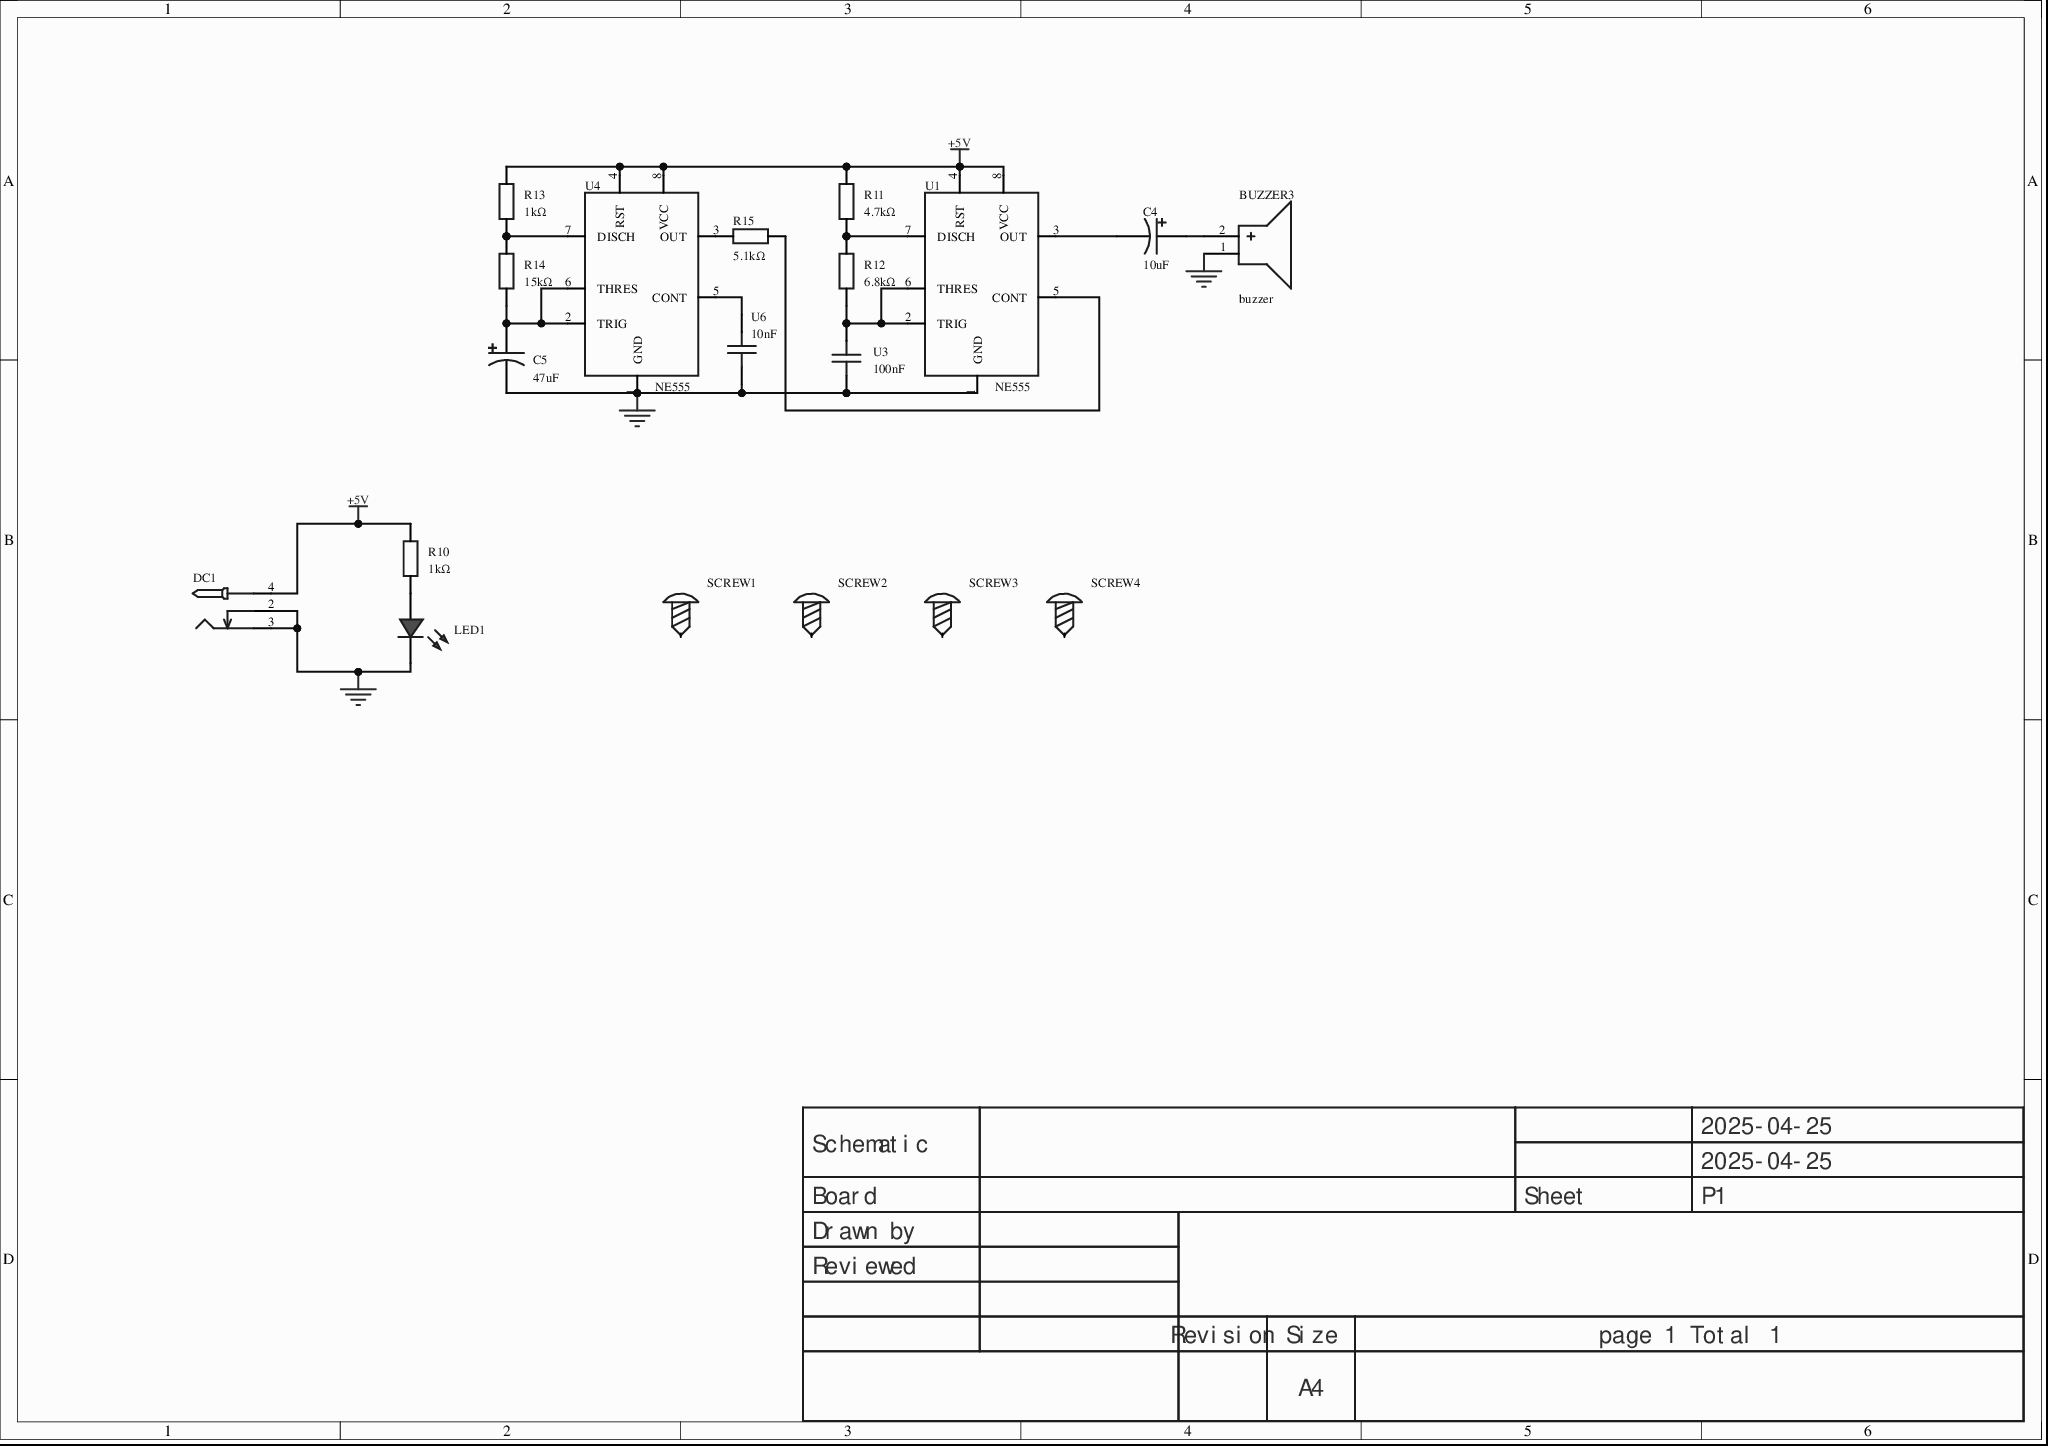
[diagram p0: MISC51829-3.schdoc]
# Altium project MISC51829-2.PrjPcb
1 sheet, 19 parts. Net scope: global (net labels, ports and power ports of the same name join across sheets).
Board file: MISC51829.pcbdoc

## Sheet MISC51829-3.schdoc
size 297 x 209 mm; Version: V1.0; @Project Name: MISC51829; @Page Count: 1; @Update Date: 2025-04-25; @Create Date: 2025-04-25; @Schematic Name: MISC51829; @Page No: 1; @Create Time: 10:10:14; @Update Time: 10:10:18; @Board Name: MISC51829

### Parts
BUZZER3  buzzer  [BUZ-TH_BD12.0-P6.00-D0.9-RD]
C4  10uF  [CAP-TH_BD5.0-P2.00-D0.8-FD]
C5  47uF  [CAP-TH_BD5.0-P2.00-D0.8-FD]
DC1  (no value)  [DC-2.0]
LED1  (no value)  [LED_TH-3mm]
R10  1kΩ  [Res_1/8W]
R11  4.7kΩ  [Res_1/8W]
R12  6.8kΩ  [Res_1/8W]
R13  1kΩ  [Res_1/8W]
R14  15kΩ  [Res_1/8W]
R15  5.1kΩ  [Res_1/8W]
SCREW1  (no value)  [M3螺丝]
SCREW2  (no value)  [M3螺丝]
SCREW3  (no value)  [M3螺丝]
SCREW4  (no value)  [M3螺丝]
U1  NE555  [PDIP-8_L9.6-W6.4-P2.54-LS7.9-BL-1]
U3  100nF  [CAP-TH_L4.0-W2.5-P2.50-D0.5]
U4  NE555  [PDIP-8_L9.6-W6.4-P2.54-LS7.9-BL-1]
U6  10nF  [CAP-TH_L4.0-W2.5-P2.50-D0.5]

### Nets
+5V: DC1.4 R10.2 R11.2 R13.2 U1.4(RST) U1.8(VCC) U4.4(RST) U4.8(VCC)
GND: BUZZER3.1(-) C5.2 DC1.2 DC1.3 LED1.2(A) U1.1(GND) U3.1 U4.1(GND) U6.1
NetBUZZER3_2: BUZZER3.2(+) C4.1
NetC4_2: C4.2 U1.3(OUT)
NetC5_1: C5.1 R14.1 U4.2(TRIG) U4.6(THRES)
NetLED1_1: LED1.1(C) R10.1
NetR11_1: R11.1 R12.2 U1.7(DISCH)
NetR12_1: R12.1 U1.2(TRIG) U1.6(THRES) U3.2
NetR13_1: R13.1 R14.2 U4.7(DISCH)
NetR15_1: R15.1 U1.5(CONT)
NetR15_2: R15.2 U4.3(OUT)
NetU4_5: U4.5(CONT) U6.2

Not connected (* = marked no-connect by the designer): SCREW1 1; SCREW2 1; SCREW3 1; SCREW4 1

### Notes on the sheet
- 2025-04-25
- Schematic
- Board
- Sheet
- P1
- Drawn by
- Reviewed
- Revision
- Size
- A4
- page 1 Total 1

### Library data of the parts
BUZZER3 = buzzer: AddInBom: yes; ModelId: af17e4151ed84fc2a628230bf2376363; ModelTransform: 472.44,472.176,0,270,0,0,0,0,-196.85; Symbol: BUZZER; Device: buzzer; LCSC Part Name: buzzer; SupplierPart: C9900014030; ManufacturerPart: buzzer; Supplier Footprint: buzzer; JLCPCB Part Class: Extended library; Supplier: LCSC; ConvertToPcb: yes; FootprintName: BUZ-TH_BD12.0-P6.00-D0.9-RD; ModelName: BUZ-TH_BD12.0-P6.00-D0.9-RD
C4 C5 = KM475M100D11RR0VH2FP0: Capacitance: 4.7uF; Tolerance: ±20%; Rated voltage: 100V;; Manufacturer: CX(承兴); Symbol: 4.7uF 100V 5*11; AddInBom: yes; ModelId: edeeed87cbc746108d01291548c38636; ModelName: CAP-TH_D5.0×H7.0×P2.0; ModelTransform: 197.091,196.7911,0,0,0,0,0,0,-137.795; φD: 5mm; L: 11mm; Device: KM475M100D11RR0VH2FP0; LCSC Part Name: 4.7uF ±20% 100V; ManufacturerPart: KM475M100D11RR0VH2FP0; Supplier Footprint: 插件,D5xL11mm; JLCPCB Part Class: Extended library; Datasheet: https://atta.szlcsc.com/upload/public/pdf/source/20211027/06D6BA3719C264B639DC286D935D03EA.pdf; Supplier: LCSC; ConvertToPcb: yes; FootprintName: CAP-TH_BD5.0-P2.00-D0.8-FD; Rated Voltage: 100V; Lead Spacing: 2mm; Lifetime @ Temp: -
  C4: Value: 10uF
  C5: Value: 47uF
DC1 = DC-005_2.0: ConvertToPcb: yes; SymbolName: DC power jack; ModelId: f5f20b8a2308479b936ba3c2698865bb0819f05c4eef4c71ace90d822a990e87; ModelName: DC-IN-TH_DC-5520-1; ModelTransform: 372.05,551.18,582.68,90,0,0,137.8,0,-149.61; Device: DC-005_2.0; AddInBom: yes; Supplier Footprint: 插件; FootprintName: DC-2.0
LED1 = LED_TH-R_3mm: ConvertToPcb: yes; ModelId: a497c992633541038a38947cdc58012f; ModelName: LED-TH-3mm_R; ModelTransform: 141.274,153.327,0,0,0,0,-5.984,0,-137.795; Symbol: LED_TH-R; Device: LED_TH-R_3mm; AddInBom: yes; FootprintName: LED_TH-3mm; Supplier Footprint: 插件
R10-R15 = Res_AXIAL-1/8W: ConvertToPcb: yes; SymbolName: Resistor; ModelId: b2b5ae7ae4c642178fe0039925c86a3f; ModelName: RES-TH_BD1.8-L3.2-P7.20-D0.4; ModelTransform: 282.86,66.88,253.09,0,0,0,0,0,-191; Device: Res_AXIAL-1/8W; AddInBom: yes; Supplier Footprint: 轴向引线; FootprintName: Res_1/8W
  R10 R13: Value: 1kΩ
  R11: Value: 4.7kΩ
  R12: Value: 6.8kΩ
  R14: Value: 15kΩ
  R15: Value: 5.1kΩ
SCREW1-SCREW4 = M3螺丝: Device: M3 screw; ConvertToPcb: yes; SymbolName: Screw hole; AddInBom: yes; Supplier Footprint: 插件; FootprintName: M3 screw
U1 U4 = NE555PE4: NE555 single timer; Manufacturer: TI(德州仪器); AddInBom: yes; ModelId: 1b8eaf096e7944deafe216467068c10e; ModelTransform: 377.952,318.897,0,0,0,0,0,0,-118.11; Manufacturer Part: NE555; Symbol: NE555PE4; Device: NE555PE4; LCSC Part Name: NE555PE4; SupplierPart: C2859604; Supplier Footprint: PDIP-8; JLCPCB Part Class: Extended library; Datasheet: https://www.ti.com/cn/lit/gpn/sa555; Supplier: LCSC; ConvertToPcb: yes; FootprintName: PDIP-8_L9.6-W6.4-P2.54-LS7.9-BL-1; ModelName: PDIP-8_L9.6-W6.4-P2.54-LS7.9-BL-1
U3 U6 = FK18X7R1H103K: Capacitance: 10nF; Tolerance: ±10%; Rated voltage: 50V; Temperature coefficient: X7R;; Manufacturer: TDK; AddInBom: yes; ModelId: 29f34a7a495a447ab8bf96a7f673455e; ModelTransform: 189.7897,98.8187,0,0,0,0,0,0,-196.85; Symbol: FK18X7R1H103K; Device: FK18X7R1H103K; LCSC Part Name: 10nF ±10% 50V; ManufacturerPart: FK18X7R1H103K; Supplier Footprint: -; JLCPCB Part Class: Extended library; Supplier: LCSC; ConvertToPcb: yes; FootprintName: CAP-TH_L4.0-W2.5-P2.50-D0.5; ModelName: CAP-TH_L4.0-W2.5-P2.50-D0.5; Voltage Rated: 50V; Temperature Coefficient: X7R
  U3: Value: 100nF
  U6: Value: 10nF